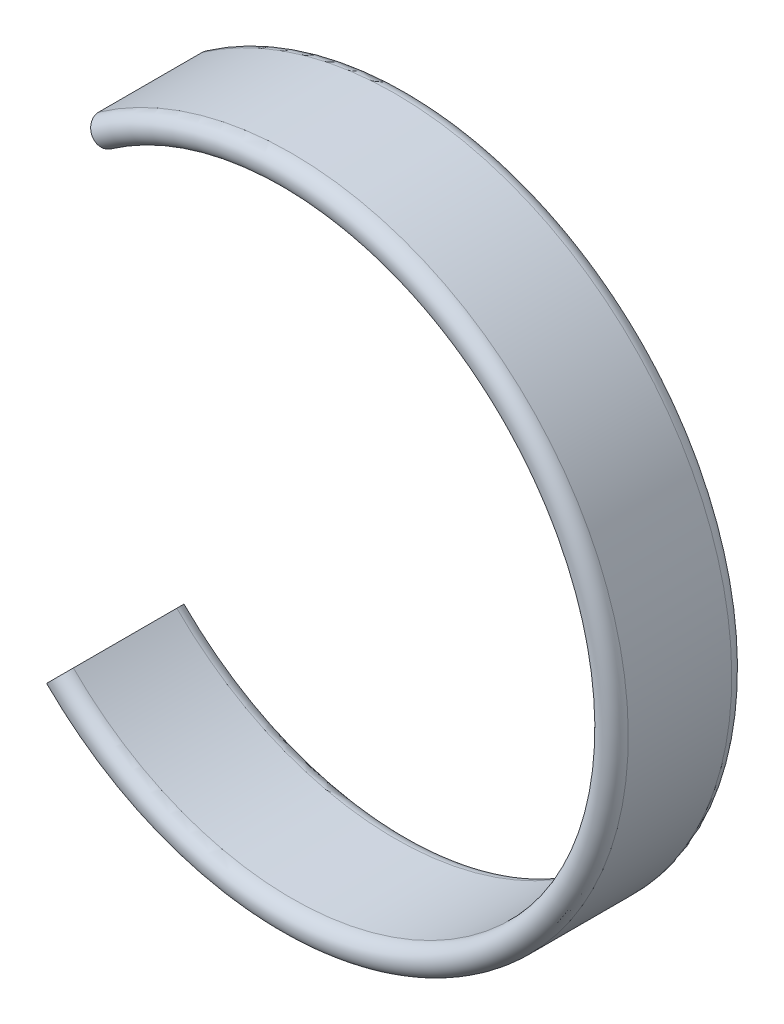
SolidWorks part; units mm, degrees
ref_plane "Front plane" through (0, 0, 0) normal (0, 0, 1) x (1, 0, 0)
ref_plane "Top plane" through (0, 0, 0) normal (0, 1, 0) x (1, 0, 0)
ref_plane "Right plane" through (0, 0, 0) normal (1, 0, 0) x (0, 0, -1)
sketch "Sketch 1" plane through (0, 0, 0) normal (0, 0, 1) x (1, 0, 0)
  line L0 (0, 0) -> (-30.0554, 42.9236) construction
  line L1 (0, 0) -> (-37.0524, -37.0524) construction
  arc A0 (-37.0524, -37.0524) -> (-30.0554, 42.9236) centre (0, 0) ccw
  dimension "D1" = 260
  dimension "D2" = 52.4
ref_plane "Reference plane 1" through (0, 0, 0) normal (0.8192, 0.5736, 0) x (-0.5736, 0.8192, 0)
sketch "Sketch 2" plane through (0, 0, 0) normal (0.8192, 0.5736, 0) x (-0.5736, 0.8192, 0)
  line L0 (52.4, -8.4) -> (52.4, 8.4) construction
  line L1 (50.45, -8.4) -> (50.45, 8.4)
  line L2 (54.35, -8.4) -> (54.35, 8.4)
  line L3 (52.4, -8.4) -> (52.4, 8.4) construction
  line L4 (50.15, -8.4) -> (50.15, 8.4)
  line L5 (54.65, -8.4) -> (54.65, 8.4)
  arc A0 (50.45, -8.4) -> (54.35, -8.4) centre (52.4, -8.4) ccw
  arc A1 (54.35, 8.4) -> (50.45, 8.4) centre (52.4, 8.4) ccw
  arc A2 (50.15, -8.4) -> (54.65, -8.4) centre (52.4, -8.4) ccw
  arc A3 (54.65, 8.4) -> (50.15, 8.4) centre (52.4, 8.4) ccw
  point P0 (52.4, 0)
  point P2 (52.4, 0)
  point P11 (52.4, 0)
  point P16 (50.45, 0)
  point P18 (52.4, -10.35)
  dimension "D2" = 10.35
  dimension "D1" = 0.3
  dimension "D4" = 1.95
sweep "Sweep 2" add profiles "Sketch 2" path "Sketch 1"
